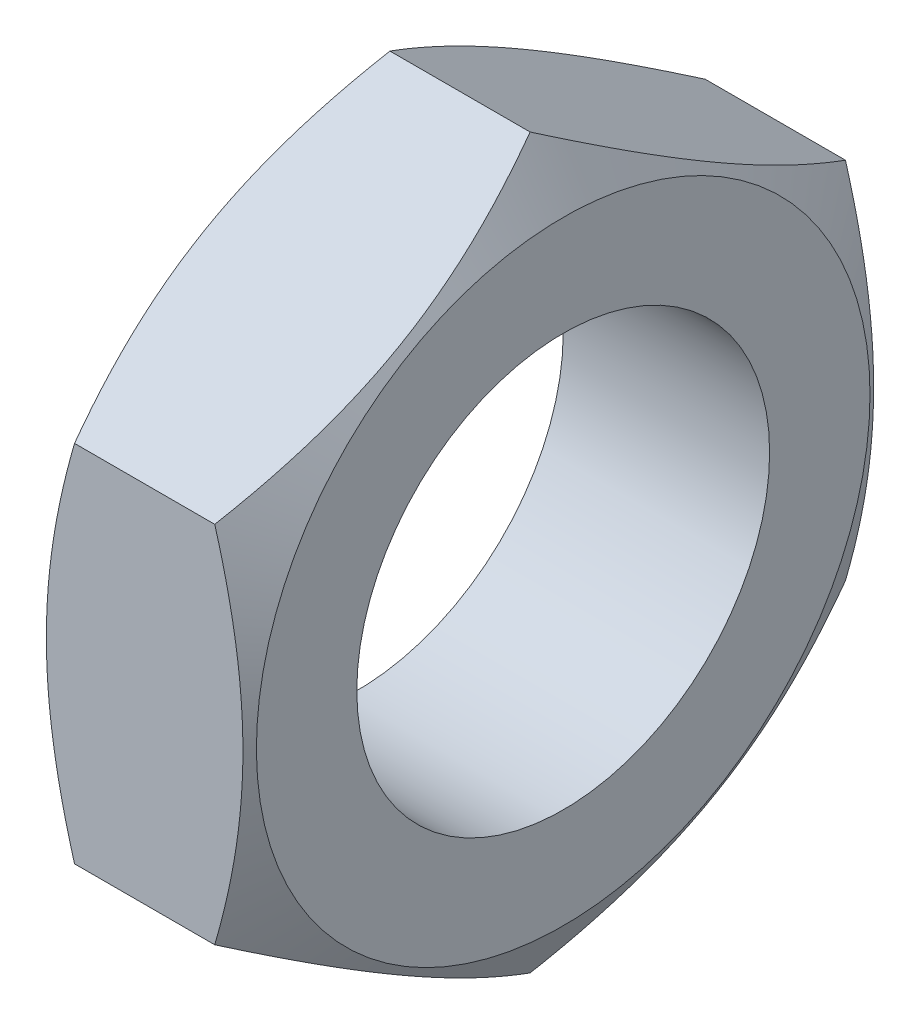
from build123d import *

# Parameters (mm, degrees)
EXTRUDE1_DEPTH      = 9
EXTRUDE1_DEPTH_BACK = 9


with BuildPart() as part:
    # Sketch1 → Extrude1 (new, two sides: drawn at the far end of the back side and taken through both)
    with BuildSketch(Plane(origin=(0, 0, 0), x_dir=(0, 0, -1), z_dir=(1, 0, 0)).offset(-EXTRUDE1_DEPTH_BACK)):
        Polygon((0, -31.754264805), (27.5, -15.877132403), (27.5, 15.877132403), (0, 31.754264805), (-27.5, 15.877132403), (-27.5, -15.877132403), align=None)
    extrude(amount=EXTRUDE1_DEPTH + EXTRUDE1_DEPTH_BACK)

    # Sketch4 → M36x2.0 Tapped Hole1 (revolve, cut)
    with BuildSketch(Plane(origin=(-9, 0, 0), x_dir=(0, 0, 1), z_dir=(0, 1, 0))):
        Polygon((0, 0), (0, 88.214630523), (17, 78), (17, 72), (18, 72), (18, 0), align=None)
    revolve(axis=Axis((-15.35, 0, 0), (1, 0, 0)), mode=Mode.SUBTRACT)

    # Sketch2 → Cut-Revolve1 (revolve, cut)
    with BuildSketch(Plane.XY, mode=Mode.PRIVATE) as cut_revolve1_sk:
        Polygon((9, 31.754264805), (6.113248654, 31.754264805), (9, 26.754264805), align=None)
    cut_revolve1 = revolve(cut_revolve1_sk.sketch.rotate(Axis((-9, 0, 0), (-1, 0, 0)), 240.000000138), axis=Axis((-9, 0, 0), (-1, 0, 0)), mode=Mode.SUBTRACT)

    # Mirror1: Cut-Revolve1 across plane
    add(cut_revolve1.mirror(Plane(origin=(0, 0, 0), x_dir=(0, 0, 1), z_dir=(1, 0, 0))), mode=Mode.SUBTRACT)


solid = part.part
